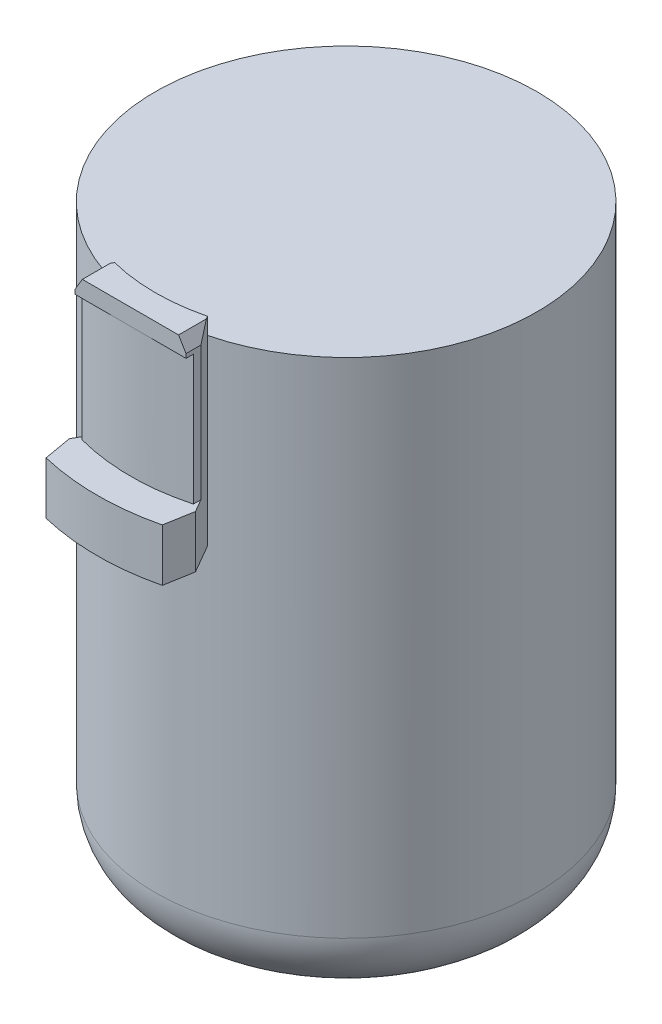
from build123d import *

# Parameters (mm, degrees)
EXTRUDE_1_DEPTH     = 15.65
EXTRUDE_2_DEPTH     = 2
CUT_EXTRUDE_1_DEPTH = 28
EXTRUDE_3_DEPTH     = 6.31


with BuildPart() as part:
    # 草图1 → 旋转1 (revolve)
    with BuildSketch(Plane.XY, mode=Mode.PRIVATE) as revolve_1_sk:
        with BuildLine():
            Line((0, -31.8), (23, -31.8))
            Line((23, -31.8), (23, -92.431634433))
            ThreePointArc((23, -92.431634433), (21.346826722, -97.301725865), (17.070552361, -100.159041043))
            Line((17.070552361, -100.159041043), (10.2, -102))
            Line((10.2, -102), (7.85, -102))
            Line((7.85, -102), (7.85, -104.1))
            Line((7.85, -104.1), (0, -104.1))
            Line((0, -104.1), (0, -31.8))
        make_face()
    revolve(revolve_1_sk.sketch.rotate(Axis((0, -104.1, 0), (0, 1, 0)), 270), axis=Axis((0, -104.1, 0), (0, 1, 0)))

    # 草图2 → 凸台-拉伸1 (add)
    with BuildSketch(Plane(origin=(0, -31.8, 0), x_dir=(1, 0, 0), z_dir=(0, 1, 0))):
        with BuildLine():
            Line((6.7, -25.121902794), (6.7, -24.206154273))
            Line((6.7, -24.206154273), (5.541103538, -22.19888672))
            ThreePointArc((5.541103538, -22.19888672), (0, -22.88), (-5.541103538, -22.19888672))
            Line((-5.541103538, -22.19888672), (-6.7, -24.206154273))
            Line((-6.7, -24.206154273), (-6.7, -25.121902794))
            ThreePointArc((-6.7, -25.121902794), (0, -26), (6.7, -25.121902794))
        make_face()
    extrude(amount=-EXTRUDE_1_DEPTH)

    # 草图3 → 凸台-拉伸2 (add)
    with BuildSketch(Plane(origin=(0, -31.8, 0), x_dir=(1, 0, 0), z_dir=(0, 1, 0))):
        with BuildLine():
            Line((-6.7, -26), (6.7, -26))
            Line((6.7, -26), (6.7, -24.206154273))
            Line((6.7, -24.206154273), (5.60350337, -22.3069664))
            ThreePointArc((5.60350337, -22.3069664), (0, -23), (-5.60350337, -22.3069664))
            Line((-5.60350337, -22.3069664), (-6.7, -24.206154273))
            Line((-6.7, -24.206154273), (-6.7, -26))
        make_face()
    extrude(amount=EXTRUDE_2_DEPTH)

    # 草图4 → 切除-拉伸1 (cut)
    with BuildSketch(Plane.XY):
        Polygon((-7, -31.8), (-5.798278762, -29.8), (5.798278762, -29.8), (7, -31.8), (7, -27.8), (-7, -27.8), align=None)
    extrude(amount=CUT_EXTRUDE_1_DEPTH, mode=Mode.SUBTRACT)

    # 草图5 → 凸台-拉伸3 (add)
    with BuildSketch(Plane(origin=(0, -47.45, 0), x_dir=(1, 0, 0), z_dir=(0, 1, 0))):
        with BuildLine():
            Line((-7.6, -25.765), (-7.004357404, -29.170858358))
            ThreePointArc((-7.004357404, -29.170858358), (0, -30), (7.004357404, -29.170858358))
            Line((7.004357404, -29.170858358), (7.6, -25.765))
            Line((7.6, -25.765), (5.541103538, -22.19888672))
            ThreePointArc((5.541103538, -22.19888672), (0, -22.88), (-5.541103538, -22.19888672))
            Line((-5.541103538, -22.19888672), (-7.6, -25.765))
        make_face()
    extrude(amount=-EXTRUDE_3_DEPTH)


solid = part.part
